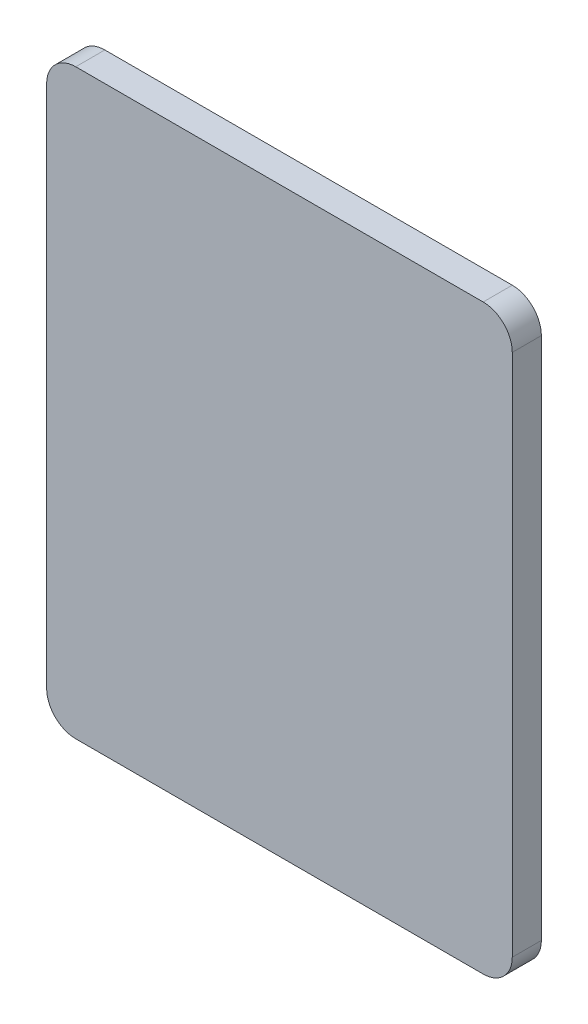
SolidWorks part; units mm, degrees
material "普通碳钢"
ref_plane "Front Plane" through (0, 0, 0) normal (0, 0, 1) x (1, 0, 0)
ref_plane "Top Plane" through (0, 0, 0) normal (0, 1, 0) x (1, 0, 0)
ref_plane "Right Plane" through (0, 0, 0) normal (1, 0, 0) x (0, 0, -1)
sketch "Sketch1" plane through (0, 0, 0) normal (0, 0, 1) x (1, 0, 0)
  line L0 (-7.1673, -80) -> (100.5878, -80) construction
  line L1 (0, 0) -> (80, 0)
  line L2 (0, 0) -> (0, -100)
  line L3 (0, -100) -> (80, -100)
  line L4 (80, 0) -> (80, -100)
  line L5 (0, 0) -> (80, -100) construction
  line L6 (0, -100) -> (80, 0) construction
  point P6 (40, -50)
  dimension "D1" = 80
  dimension "D2" = 100
  dimension "D4" = 80
extrude "Boss-Extrude1" add sketch "Sketch1" along normal blind 5
fillet "Fillet1" radius 5 4 edges at (80, -100, 2.5) (0, -100, 2.5) (80, 0, 2.5) (0, 0, 2.5)
